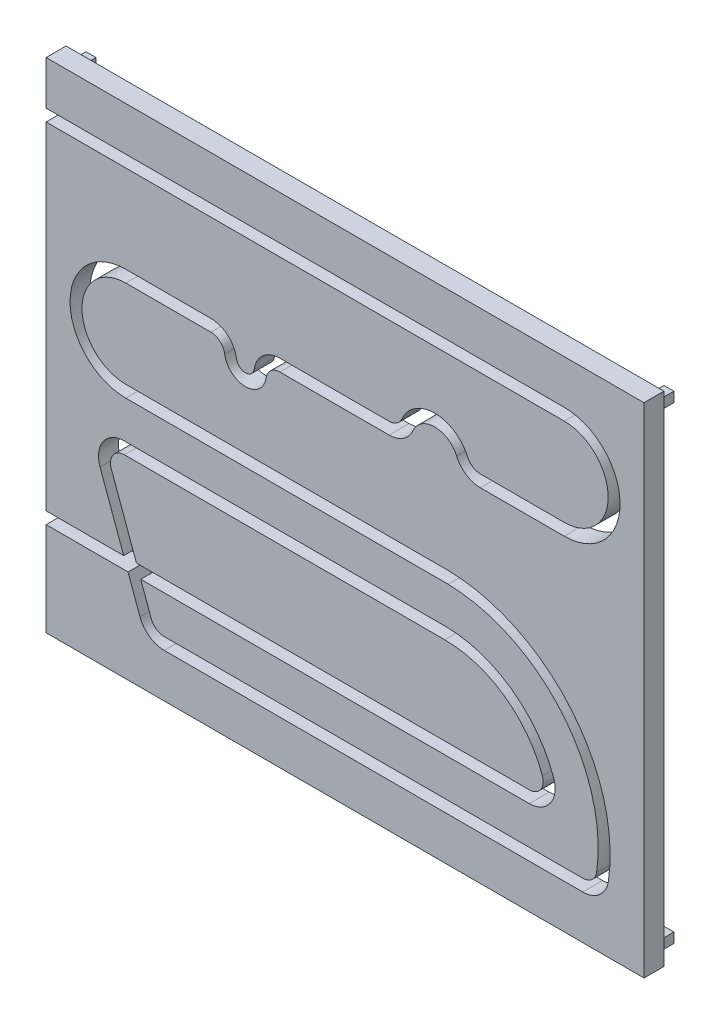
from build123d import *

# Parameters (mm, degrees)
SKETCH1_W                    = 600
SKETCH1_H                    = 500
BOSS_EXTRUDE1_DEPTH          = 20
CUT_EXTRUDE_THIN1_DEPTH      = 392.02429592
CUT_EXTRUDE_THIN1_DEPTH_BACK = 20
CUT_EXTRUDE_THIN2_DEPTH      = 392.02429592
CUT_EXTRUDE_THIN2_DEPTH_BACK = 20
SKETCH3_W                    = 484.852813742
SKETCH3_H                    = 12
SKETCH4_W                    = 10
SKETCH4_H                    = 10
BOSS_EXTRUDE2_DEPTH          = 15
MIRROR2_COPY_1_SKETCH_W      = 10
MIRROR2_COPY_1_SKETCH_H      = 10
MIRROR2_COPY_1_DEPTH         = 15


with BuildPart() as part:
    # Sketch1 → Boss-Extrude1 (new body)
    with BuildSketch(Plane.XY):
        Rectangle(SKETCH1_W, SKETCH1_H)
    extrude(amount=BOSS_EXTRUDE1_DEPTH)

    # Sketch2 → Cut-Extrude-Thin1 (cut, two sides: drawn at the far end of the back side and taken through both)
    with BuildSketch(Plane.XY.offset(20).offset(-CUT_EXTRUDE_THIN1_DEPTH_BACK)):
        with BuildLine():
            Line((-300, 193.961076205), (220, 193.961076205))
            ThreePointArc((220, 193.961076205), (264, 149.961076205), (220, 105.961076205))
            Line((220, 105.961076205), (135.82575695, 105.961076205))
            ThreePointArc((135.82575695, 105.961076205), (128.157641144, 108.247835834), (122.994545004, 114.361076205))
            ThreePointArc((122.994545004, 114.361076205), (90, 135.961076205), (57.005454996, 114.361076205))
            ThreePointArc((57.005454996, 114.361076205), (51.842358856, 108.247835834), (44.17424305, 105.961076205))
            Line((44.17424305, 105.961076205), (-2.040587873, 105.961076205))
            Line((-2.040587873, 105.961076205), (-65.358983849, 105.961076205))
            ThreePointArc((-65.358983849, 105.961076205), (-82.379979287, 99.615228802), (-91.092310133, 83.675361919))
            ThreePointArc((-91.092310133, 83.675361919), (-100, 75.961076205), (-108.907689867, 83.675361919))
            ThreePointArc((-108.907689867, 83.675361919), (-117.620020713, 99.615228802), (-134.641016151, 105.961076205))
            Line((-134.641016151, 105.961076205), (-220, 105.961076205))
            ThreePointArc((-220, 105.961076205), (-276, 49.961076205), (-220, -6.038923795))
            Line((-220, -6.038923795), (103.462226705, -6.038923795))
            ThreePointArc((103.462226705, -6.038923795), (217.539052876, -60.498386701), (252.420471066, -182))
            ThreePointArc((252.420471066, -182), (247.729215995, -190.583005244), (238.564064606, -194))
            Line((238.564064606, -194), (-181.400314096, -194))
            ThreePointArc((-181.400314096, -194), (-189.430384205, -191.46812862), (-194.556010787, -184.788282007))
            Line((-194.556010787, -184.788282007), (-234.592736556, -74.788282007))
            ThreePointArc((-234.592736556, -74.788282007), (-232.905168485, -61.969929891), (-221.437039865, -56))
            Line((-221.437039865, -56), (100, -56))
            ThreePointArc((100, -56), (160.044427996, -75.084355584), (198.052140325, -125.333333333))
            ThreePointArc((198.052140325, -125.333333333), (196.283765875, -138.082903769), (184.852813742, -144))
            Line((184.852813742, -144), (184.852813742, -156))
            ThreePointArc((184.852813742, -156), (206.081724847, -145.011106999), (209.365848824, -121.333333333))
            ThreePointArc((209.365848824, -121.333333333), (166.972631226, -65.286396612), (100, -44))
            Line((100, -44), (-221.437039865, -44))
            ThreePointArc((-221.437039865, -44), (-242.734993017, -55.087012655), (-245.869048006, -78.892523726))
            Line((-245.869048006, -78.892523726), (-205.832322236, -188.892523726))
            ThreePointArc((-205.832322236, -188.892523726), (-196.313301441, -201.297953152), (-181.400314096, -206))
            Line((-181.400314096, -206), (238.564064606, -206))
            ThreePointArc((238.564064606, -206), (255.585060044, -199.654152596), (264.297390889, -183.714285714))
            ThreePointArc((264.297390889, -183.714285714), (226.653528564, -52.692573871), (103.594604963, 5.961076205))
            Line((103.594604963, 5.961076205), (-220, 5.961076205))
            ThreePointArc((-220, 5.961076205), (-264, 49.961076205), (-220, 93.961076205))
            Line((-220, 93.961076205), (-134.641016151, 93.961076205))
            ThreePointArc((-134.641016151, 93.961076205), (-125.475864761, 90.544081449), (-120.784609691, 81.961076205))
            ThreePointArc((-120.784609691, 81.961076205), (-100, 63.961076205), (-79.215390309, 81.961076205))
            ThreePointArc((-79.215390309, 81.961076205), (-74.524135239, 90.544081449), (-65.358983849, 93.961076205))
            Line((-65.358983849, 93.961076205), (-2.040587873, 93.961076205))
            Line((-2.040587873, 93.961076205), (44.17424305, 93.961076205))
            ThreePointArc((44.17424305, 93.961076205), (58.415029546, 98.207915515), (68.003636664, 109.561076205))
            ThreePointArc((68.003636664, 109.561076205), (90, 123.961076205), (111.996363336, 109.561076205))
            ThreePointArc((111.996363336, 109.561076205), (121.584970454, 98.207915515), (135.82575695, 93.961076205))
            Line((135.82575695, 93.961076205), (220, 93.961076205))
            ThreePointArc((220, 93.961076205), (276, 149.961076205), (220, 205.961076205))
            Line((220, 205.961076205), (-300, 205.961076205))
            Line((-300, 205.961076205), (-300, 193.961076205))
        make_face()
    extrude(amount=CUT_EXTRUDE_THIN1_DEPTH + CUT_EXTRUDE_THIN1_DEPTH_BACK, mode=Mode.SUBTRACT)

    # Sketch3 → Cut-Extrude-Thin2 (cut, two sides: drawn at the far end of the back side and taken through both)
    with BuildSketch(Plane.XY.offset(20).offset(-CUT_EXTRUDE_THIN2_DEPTH_BACK)):
        with Locations((-57.573593129, -150)):
            Rectangle(SKETCH3_W, SKETCH3_H)
    extrude(amount=CUT_EXTRUDE_THIN2_DEPTH + CUT_EXTRUDE_THIN2_DEPTH_BACK, mode=Mode.SUBTRACT)


with BuildPart() as cut_extrude_thin2_piece_1:
    # of the separate pieces the step leaves, piece 1, a body of its own (cut_extrude_thin2_pieces)
    add(part.part.solids().sort_by_distance((-300, 250, 0))[0])

    # Sketch4 → Boss-Extrude2 (add)
    with BuildSketch(Plane(origin=(0, 0, 0), x_dir=(-1, 0, 0), z_dir=(0, 0, -1))):
        with Locations((-290, 235)):
            Rectangle(SKETCH4_W, SKETCH4_H)
    boss_extrude2 = extrude(amount=BOSS_EXTRUDE2_DEPTH)

    # Mirror1: Boss-Extrude2 across plane
    add(boss_extrude2.mirror(Plane(origin=(0, 0, 0), x_dir=(0, 0, 1), z_dir=(1, 0, 0))))

    # Mirror2: Boss-Extrude2 across plane
    add(boss_extrude2.mirror(Plane.ZX))

    # Mirror2 copy 1 sketch → Mirror2 copy 1 (add)
    with BuildSketch(Plane(origin=(0, 0, 0), x_dir=(1, 0, 0), z_dir=(0, 0, -1))):
        with Locations((-290, 235)):
            Rectangle(MIRROR2_COPY_1_SKETCH_W, MIRROR2_COPY_1_SKETCH_H)
    extrude(amount=MIRROR2_COPY_1_DEPTH)


with BuildPart() as cut_extrude_thin2_piece_2:
    # of the separate pieces the step leaves, piece 2, a body of its own (cut_extrude_thin2_pieces)
    add(part.part.solids().sort_by_distance((-222.171864614, -144, 0))[0])


with BuildPart() as cut_extrude_thin2_piece_3:
    # of the separate pieces the step leaves, piece 3, a body of its own (cut_extrude_thin2_pieces)
    add(part.part.solids().sort_by_distance((198.052140325, -125.333333333, 0))[0])


solid = Compound([cut_extrude_thin2_piece_1.part, cut_extrude_thin2_piece_2.part, cut_extrude_thin2_piece_3.part])
